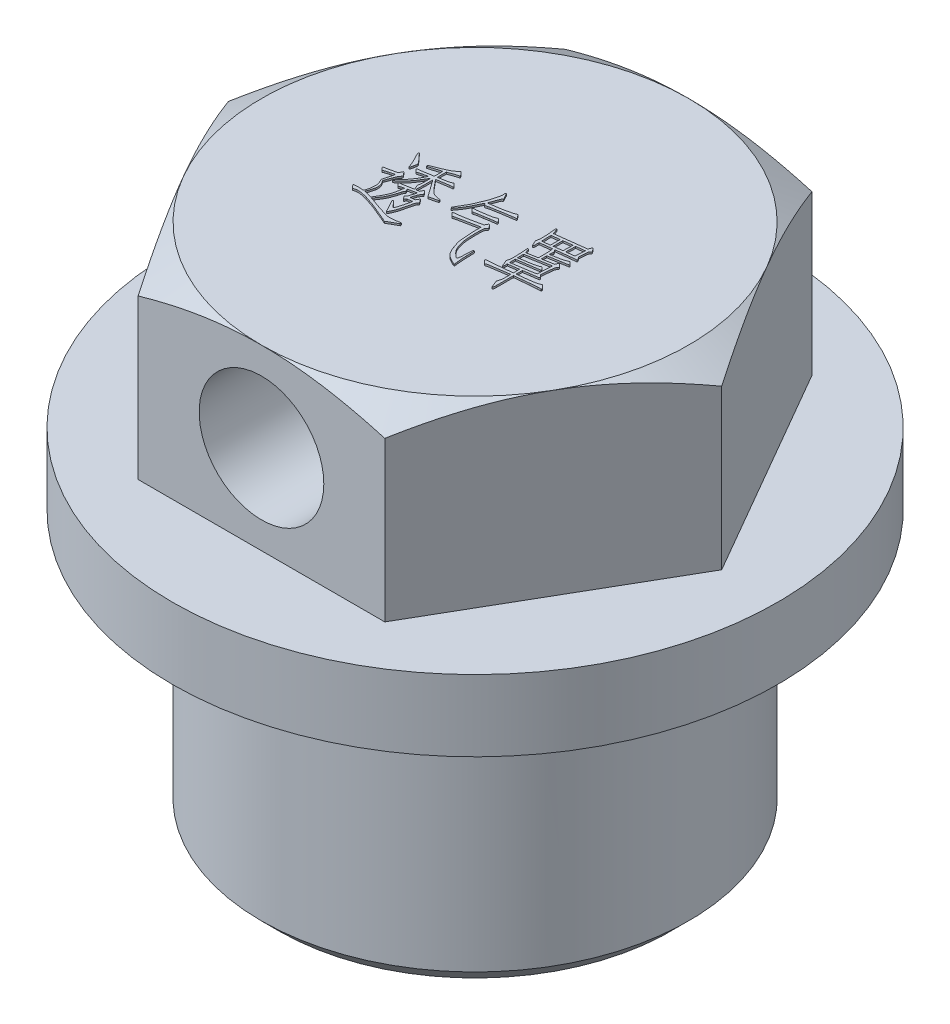
SolidWorks part; units mm, degrees
ref_plane "Front Plane" through (0, 0, 0) normal (0, 0, 1) x (1, 0, 0)
ref_plane "Top Plane" through (0, 0, 0) normal (0, 1, 0) x (1, 0, 0)
ref_plane "Right Plane" through (0, 0, 0) normal (1, 0, 0) x (0, 0, -1)
sketch "Sketch1" plane through (0, 0, 0) normal (0, 1, 0) x (1, 0, 0)
  line L1 (13.85, 0) -> (6.925, 11.9945)
  line L2 (6.925, 11.9945) -> (-6.925, 11.9945)
  line L3 (-6.925, 11.9945) -> (-13.85, 0)
  line L4 (-13.85, 0) -> (-6.925, -11.9945)
  line L5 (-6.925, -11.9945) -> (6.925, -11.9945)
  line L6 (6.925, -11.9945) -> (13.85, 0)
  circle A0 centre (0, 0) radius 11.9945 construction
  dimension "D1" = 27.7
extrude "Boss-Extrude1" add sketch "Sketch1" along normal blind 10
sketch "Sketch3" plane through (0, 0, 0) normal (1, 0, 0) x (0, 0, -1)
  line L0 (-11.9945, 10) -> (-16.6355, 10)
  line L1 (-16.6355, 10) -> (-16.6355, 7.3205)
  line L2 (-16.6355, 7.3205) -> (-11.9945, 10)
  line L3 (-11.9945, 10) -> (0, 10) construction
  line L4 (0, 0) -> (0, 17.3403) construction
  dimension "D1" = 30
revolve "Cut-Revolve1" cut sketch "Sketch3" angle 360 about L4
sketch "Sketch4" plane through (0, 0, 0) normal (0, 0, 1) x (1, 0, 0)
  line L0 (0, 0) -> (-17, 0)
  line L1 (-17, 0) -> (-17, -4)
  line L2 (-17, -4) -> (-10.85, -4)
  line L3 (-10.85, -4) -> (-10.85, -7)
  line L4 (-10.85, -7) -> (-12, -7)
  line L5 (-12, -7) -> (-12, -19)
  line L6 (-12, -19) -> (0, -19)
  line L7 (0, -19) -> (0, 0)
  line L8 (0, 15.4376) -> (0, 0) construction
  dimension "D1" = 34
  dimension "D2" = 24
  dimension "D3" = 4
  dimension "D4" = 15
  dimension "D5" = 21.7
  dimension "D6" = 3
revolve "Revolve1" add sketch "Sketch4" angle 360 about L8
cosmetic thread "Cosmetic Thread1" parameters "D2"=20.4
sketch "Sketch5" plane through (0, 0, 0) normal (0, 0, 1) x (1, 0, 0)
  line L0 (0, -19) -> (0, 9.0207)
  line L1 (-12, -19) -> (12, -19) construction
  line L2 (0, 9.0207) -> (3.5, 7)
  line L3 (3.5, 7) -> (3.5, -19)
  line L4 (3.5, -19) -> (0, -19)
  dimension "D1" = 3.5
  dimension "D2" = 60
  dimension "D3" = 26
revolve "Cut-Revolve2" cut sketch "Sketch5" angle 360 about L0
sketch "Sketch6" plane through (0, 0, 11.9945) normal (0, 0, 1) x (1, 0, 0)
  circle A0 centre (0, 5) radius 3.5
  dimension "D1" = 7
  dimension "D2" = 5
extrude "Cut-Extrude1" cut sketch "Sketch6" against normal through all
chamfer "Chamfer1" distance 1 angle 45 1 edges at (0, -19, 12)
sketch "Sketch7" plane through (0, 10, 0) normal (0, 1, 0) x (1, 0, 0)
  line L0 (-9.1019, -1.9051) -> (9.3371, -1.9051) construction
  text T0 "透气罩"
extrude "Boss-Extrude2" add sketch "Sketch7" along normal blind 0.1
